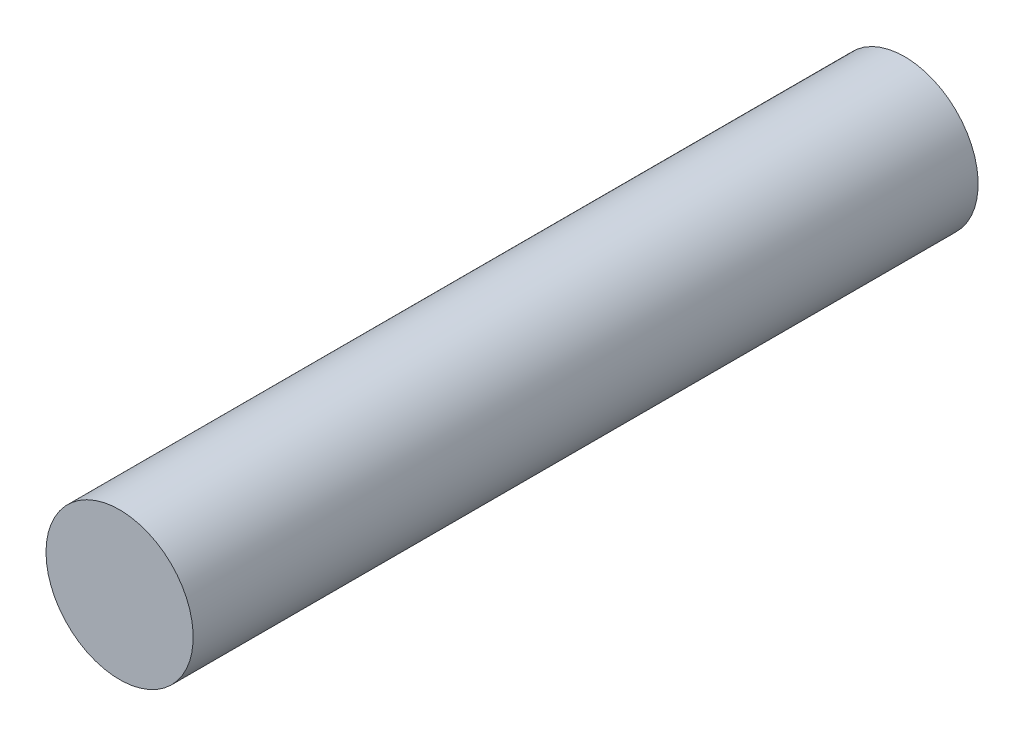
from build123d import *

# Parameters (mm, degrees)
BOSS_EXTRUDE1_DEPTH      = 20
BOSS_EXTRUDE1_DEPTH_BACK = 140
SKETCH1_R                = 15


with BuildPart() as part:
    # Sketch1 → Boss-Extrude1 (new, two sides: drawn at the far end of the back side and taken through both)
    with BuildSketch(Plane.XY.offset(-BOSS_EXTRUDE1_DEPTH_BACK)):
        with Locations(Location((70, -13, 0), (0, 0, 180))):
            Circle(SKETCH1_R)
    extrude(amount=BOSS_EXTRUDE1_DEPTH + BOSS_EXTRUDE1_DEPTH_BACK)


solid = part.part
